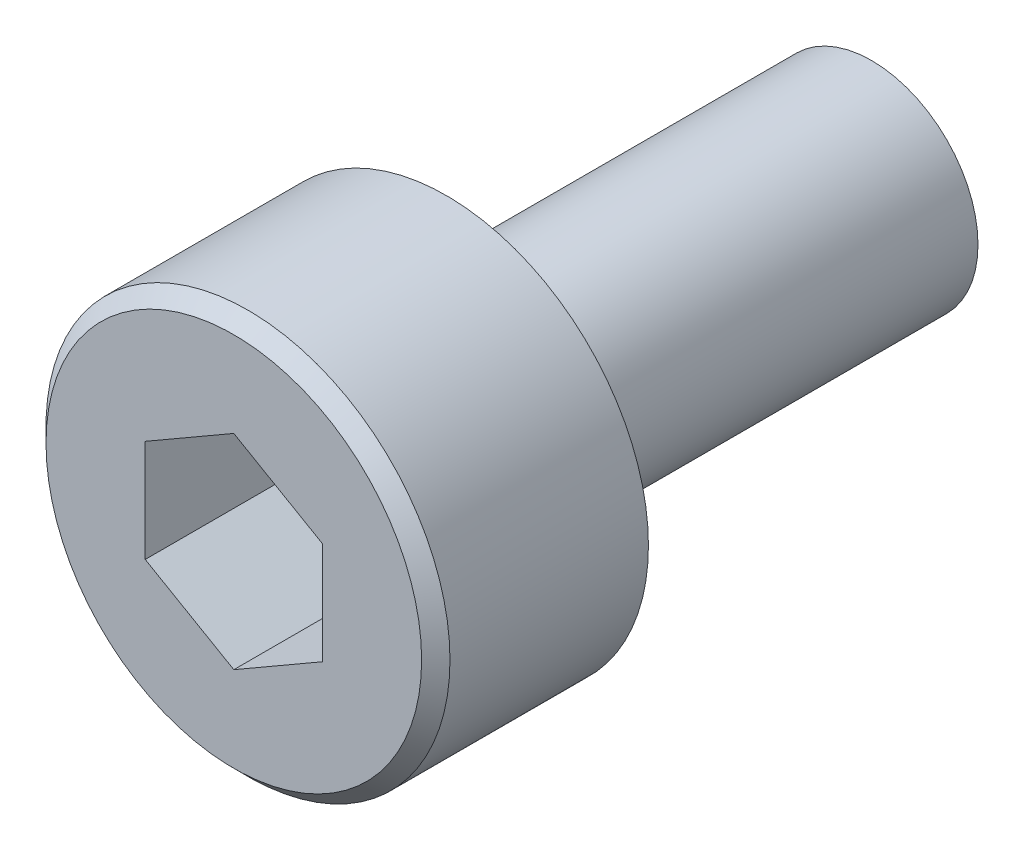
from build123d import *

# Parameters (mm, degrees)
SKETCH_1_R          = 2.85
EXTRUDE_1_DEPTH     = 3
CUT_EXTRUDE_1_DEPTH = 4
CHAMFER_1_SIZE      = 0.2
SKETCH_3_R          = 1.5
EXTRUDE_2_DEPTH     = 6


with BuildPart() as part:
    # 草图1 → 凸台-拉伸1 (new body)
    with BuildSketch(Plane.XY):
        Circle(SKETCH_1_R)
    extrude(amount=EXTRUDE_1_DEPTH)

    # 草图2 → 切除-拉伸1 (cut)
    with BuildSketch(Plane.XY.offset(3)):
        Polygon((0, 1.443375673), (-1.25, 0.721687836), (-1.25, -0.721687836), (0, -1.443375673), (1.25, -0.721687836), (1.25, 0.721687836), align=None)
    extrude(amount=-CUT_EXTRUDE_1_DEPTH, mode=Mode.SUBTRACT)

    # 倒角1
    chamfer_1_edges = [part.edges().sort_by_distance(p)[0] for p in [
        (-2.85, 0, 3),
    ]]
    chamfer(chamfer_1_edges, length=CHAMFER_1_SIZE)

    # 草图3 → 凸台-拉伸2 (add)
    with BuildSketch(Plane(origin=(0, 0, 0), x_dir=(-1, 0, 0), z_dir=(0, 0, -1))):
        with Locations(Location((0, 0, 0), (0, 0, 180))):
            Circle(SKETCH_3_R)
    extrude(amount=EXTRUDE_2_DEPTH)


solid = part.part
